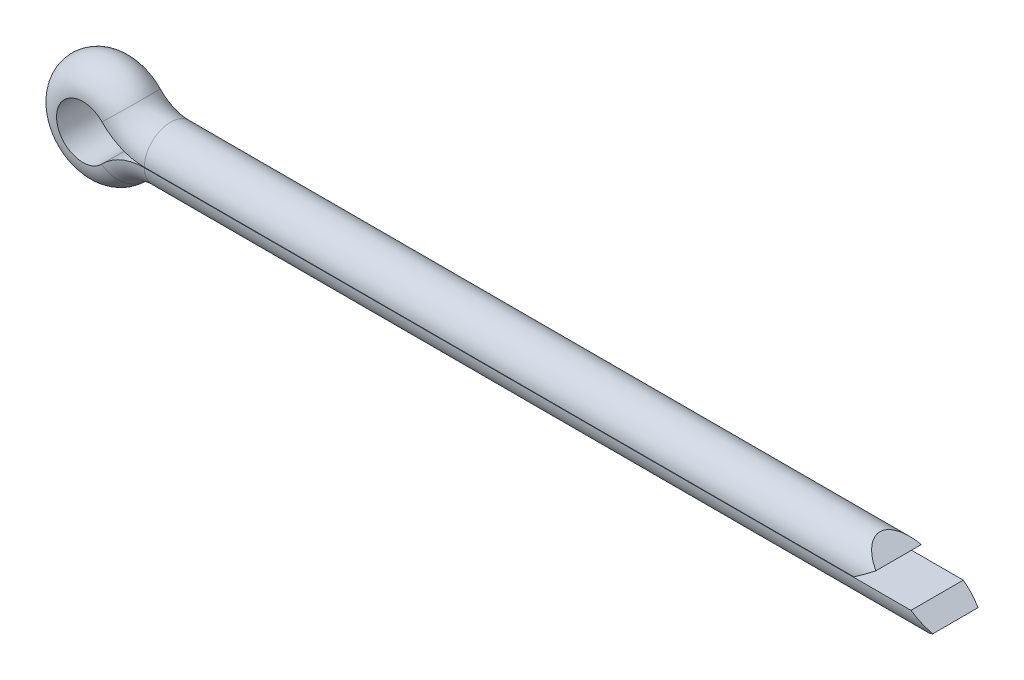
SolidWorks part; units mm, degrees
material "Q235"
ref_plane "Front Plane" through (0, 0, 0) normal (0, 0, 1) x (1, 0, 0)
ref_plane "Top Plane" through (0, 0, 0) normal (0, 1, 0) x (1, 0, 0)
ref_plane "Right Plane" through (0, 0, 0) normal (1, 0, 0) x (0, 0, -1)
sketch "Dimension Sketch" plane through (0, 0, 0) normal (0, 0, 1) x (1, 0, 0)
  line L0 (34.7, 1.15) -> (2.7, 1.15)
  line L1 (2.7, -1.15) -> (37.2, -1.15)
  line L2 (2.7, 0) -> (27.3859, 0) construction
  line L3 (2.7, 0) -> (2.7, -0.0723) construction
  line L4 (-2.3, 0) -> (-2.3, 18.8979) construction
  arc A0 (2.7, 1.15) -> (1.6584, 1.5936) centre (2.7, 2.5946) cw
  arc A1 (1.6584, 1.5936) -> (1.6584, -1.5936) centre (0, 0) ccw
  arc A2 (1.6584, -1.5936) -> (2.7, -1.15) centre (2.7, -2.5946) cw
  dimension "c" = 4.6
  dimension "d1" = 2.3
  dimension "b" = 5
  dimension "l" = 32
  dimension "a" = 2.5
ref_plane "Plane1" through (34.7, 1.15, 0) normal (-1, 0, 0) x (0, 0, 1)
sketch "Sketch2" plane through (34.7, 1.15, 0) normal (-1, 0, 0) x (0, 0, 1)
  line L0 (0, -3.45) -> (0, 1.15) construction
  line L1 (-1.15, -1.14) -> (1.15, -1.14)
  arc A0 (1.15, -1.14) -> (-1.15, -1.14) centre (0, -1.15) ccw
  dimension "d" = 2.3
  dimension "D1" = 0.01
sweep "Sweep2" add profiles "Sketch2" path "Dimension Sketch"
sketch "Sketch3" plane through (0, 0, 0) normal (0, 0, 1) x (1, 0, 0)
  line L0 (2.7, 0) -> (2.7, 16.2682) construction
  line L1 (2.7, 0) -> (37.4999, 0) construction
  line L2 (37.2, -1.15) -> (37.2, -0.01) construction
  line L3 (34.7, 0.57) -> (33.8823, 1.15)
  line L4 (34.7, 1.15) -> (2.7, 1.15) construction
  line L5 (2.7, -1.15) -> (37.2, -1.15) construction
  line L6 (34.7, 0.57) -> (33.8753, 0)
  line L7 (37.2, -0.58) -> (36.3823, 0)
  line L9 (37.2, -0.58) -> (36.3753, -1.15)
  line L10 (36.3823, 0) -> (33.8753, 0)
  line L11 (33.8823, 1.15) -> (37.21, 1.15)
  line L12 (37.21, 1.15) -> (37.21, -1.15)
  line L13 (37.21, -1.15) -> (36.3753, -1.15)
  line L14 (34.7, 1.15) -> (34.7, 0.01) construction
  dimension "D1" = 0.01
  dimension "D3" = 70
  dimension "D4" = 70
extrude "Cut-Extrude1" cut sketch "Sketch3" against normal through all and the other way through all
